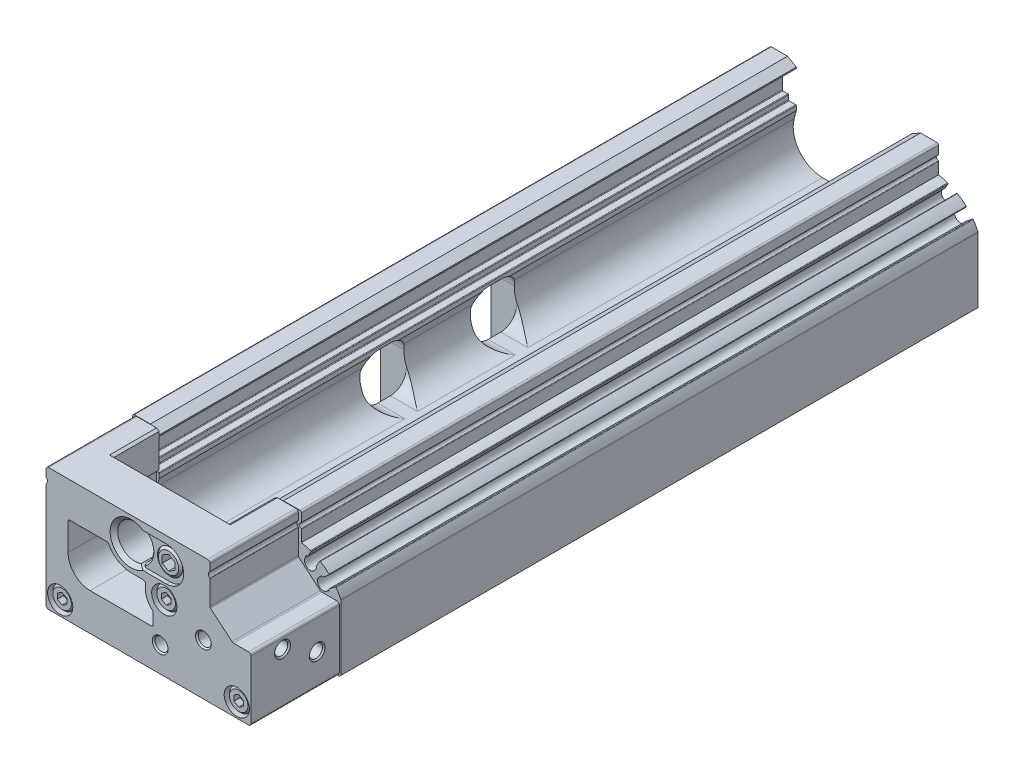
from build123d import *

# Parameters (mm, degrees)
BOSS_EXTRUDE1_DEPTH      = 28
BOSS_EXTRUDE2_DEPTH      = 202
CUT_EXTRUDE1_DEPTH       = 14.9
CUT_EXTRUDE2_DEPTH       = 8.7
BOSS_EXTRUDE3_START      = 7.5
BOSS_EXTRUDE3_DEPTH      = 7.5
BOSS_EXTRUDE4_DEPTH      = 8.7
CUT_EXTRUDE3_DEPTH       = 7.6
CUT_EXTRUDE3_DEPTH_BACK  = 7.6
CUT_EXTRUDE4_DEPTH       = 17
CUT_EXTRUDE5_DEPTH       = 7.6
CUT_EXTRUDE5_DEPTH_BACK  = 7.6
CUT_EXTRUDE6_DEPTH       = 17
CUT_EXTRUDE7_DEPTH       = 4.6
CUT_EXTRUDE7_DEPTH_BACK  = 4.6
SKETCH28_R               = 4
CUT_EXTRUDE8_DEPTH       = 4.6
CUT_EXTRUDE8_DEPTH_BACK  = 4.6
SKETCH29_R               = 4
CUT_EXTRUDE9_DEPTH       = 4.6
CUT_EXTRUDE9_DEPTH_BACK  = 4.6
SKETCH30_R               = 4
SKETCH33_W               = 8
SKETCH33_H               = 4
CUT_EXTRUDE10_DEPTH      = 5
CUT_EXTRUDE11_DEPTH      = 2
CUT_EXTRUDE11_DEPTH_BACK = 2
CUT_EXTRUDE12_DEPTH      = 2
CUT_EXTRUDE12_DEPTH_BACK = 2
CUT_EXTRUDE13_DEPTH      = 2
CUT_EXTRUDE13_DEPTH_BACK = 2


with BuildPart() as part:
    # Sketch1 → Boss-Extrude1 (new body)
    with BuildSketch(Plane.XY):
        with BuildLine():
            Line((0.8, 0), (64.2, 0))
            ThreePointArc((64.2, 0), (64.765685425, 0.234314575), (65, 0.8))
            Line((65, 0.8), (65, 19.3))
            ThreePointArc((65, 19.3), (64.765685425, 19.865685425), (64.2, 20.1))
            Line((64.2, 20.1), (59.464779164, 20.1))
            ThreePointArc((59.464779164, 20.1), (59.225365064, 20.142215165), (59.014827837, 20.26376889))
            Line((59.014827837, 20.26376889), (52.178606195, 26.000039948))
            ThreePointArc((52.178606195, 26.000039948), (52.046846106, 26.171753039), (52, 26.38306217))
            Line((52, 26.38306217), (52, 34.125320566))
            ThreePointArc((52, 34.125320566), (51.977951304, 34.216607658), (51.916666667, 34.287767138))
            ThreePointArc((51.916666667, 34.287767138), (51.5, 35.1), (51.916666667, 35.912232862))
            ThreePointArc((51.916666667, 35.912232862), (51.977951304, 35.983392342), (52, 36.074679434))
            Line((52, 36.074679434), (52, 38.2))
            ThreePointArc((52, 38.2), (51.765685425, 38.765685425), (51.2, 39))
            Line((51.2, 39), (0.8, 39))
            ThreePointArc((0.8, 39), (0.234314575, 38.765685425), (0, 38.2))
            Line((0, 38.2), (0, 36.074679434))
            ThreePointArc((0, 36.074679434), (0.022048696, 35.983392342), (0.083333333, 35.912232862))
            ThreePointArc((0.083333333, 35.912232862), (0.5, 35.1), (0.083333333, 34.287767138))
            ThreePointArc((0.083333333, 34.287767138), (0.022048696, 34.216607658), (0, 34.125320566))
            Line((0, 34.125320566), (0, 0.8))
            ThreePointArc((0, 0.8), (0.234314575, 0.234314575), (0.8, 0))
        make_face()
        with BuildLine():
            Line((7, 27.3), (7, 18.8))
            ThreePointArc((7, 18.8), (9.050252532, 13.850252532), (14, 11.8))
            Line((14, 11.8), (33.4, 11.8))
            ThreePointArc((33.4, 11.8), (33.824264069, 11.975735931), (34, 12.4))
            Line((34, 12.4), (34, 15.827959784))
            ThreePointArc((34, 15.827959784), (33.940201982, 16.089076268), (33.772727273, 16.298145258))
            ThreePointArc((33.772727273, 16.298145258), (31.893362377, 18.863270124), (31.588820692, 22.028571429))
            ThreePointArc((31.588820692, 22.028571429), (31.368943868, 22.843650304), (30.60362414, 23.2))
            Line((30.60362414, 23.2), (27, 23.2))
            ThreePointArc((27, 23.2), (22.818089899, 24.380056605), (19.869902457, 27.572093023))
            ThreePointArc((19.869902457, 27.572093023), (19.648788399, 27.811495755), (19.335145142, 27.9))
            Line((19.335145142, 27.9), (7.6, 27.9))
            ThreePointArc((7.6, 27.9), (7.175735931, 27.724264069), (7, 27.3))
        make_face(mode=Mode.SUBTRACT)
    extrude(amount=BOSS_EXTRUDE1_DEPTH)

    # Sketch2 → Boss-Extrude2 (add)
    with BuildSketch(Plane.XY):
        with BuildLine():
            Line((-0.5, 34.171291219), (-0.5, 0.25))
            Line((-0.5, 0.25), (0, -0.25))
            Line((0, -0.25), (7, -0.25))
            Line((7, -0.25), (7.25, -0.5))
            Line((7.25, -0.5), (45.15, -0.5))
            Line((45.15, -0.5), (45.4, -0.25))
            Line((45.4, -0.25), (65, -0.25))
            Line((65, -0.25), (65.5, 0.25))
            Line((65.5, 0.25), (65.5, 20.913874629))
            ThreePointArc((65.5, 20.913874629), (65.488140605, 21.022127805), (65.453125, 21.125245711))
            ThreePointArc((65.453125, 21.125245711), (64.780880489, 22.414771774), (63.997704608, 23.640098541))
            ThreePointArc((63.997704608, 23.640098541), (63.862603435, 23.723024943), (63.70959314, 23.681588675))
            Line((63.70959314, 23.681588675), (61.720720018, 22.09956756))
            ThreePointArc((61.720720018, 22.09956756), (61.646508574, 21.965686571), (61.688701313, 21.818543001))
            ThreePointArc((61.688701313, 21.818543001), (61.729316434, 21.660319143), (61.638419767, 21.524590836))
            Line((61.638419767, 21.524590836), (60.803979043, 21.001419089))
            ThreePointArc((60.803979043, 21.001419089), (58.439123592, 21.405935885), (58.576951262, 23.801176724))
            Line((58.576951262, 23.801176724), (59.274422472, 24.496542751))
            ThreePointArc((59.274422472, 24.496542751), (59.427119372, 24.554577516), (59.572151549, 24.479410735))
            ThreePointArc((59.572151549, 24.479410735), (59.706032538, 24.405199291), (59.853176108, 24.44739203))
            Line((59.853176108, 24.44739203), (61.721062189, 25.933175708))
            ThreePointArc((61.721062189, 25.933175708), (61.796411585, 26.082013006), (61.732713363, 26.236196693))
            ThreePointArc((61.732713363, 26.236196693), (60.422319434, 27.333230903), (59.00548184, 28.288839368))
            ThreePointArc((59.00548184, 28.288839368), (58.852359437, 28.311102038), (58.72918001, 28.217459497))
            Line((58.72918001, 28.217459497), (57.649038106, 26.346598839))
            ThreePointArc((57.649038106, 26.346598839), (57.629058021, 26.19483503), (57.722243186, 26.073393759))
            ThreePointArc((57.722243186, 26.073393759), (57.818021446, 25.941064993), (57.783194182, 25.781467252))
            Line((57.783194182, 25.781467252), (57.198558959, 24.988875518))
            ThreePointArc((57.198558959, 24.988875518), (54.85, 24.498522628), (54.10037858, 26.777610794))
            Line((54.10037858, 26.777610794), (54.494465545, 27.680215616))
            ThreePointArc((54.494465545, 27.680215616), (54.615267611, 27.790175782), (54.777756814, 27.773393759))
            ThreePointArc((54.777756814, 27.773393759), (54.929520623, 27.753413674), (55.050961894, 27.846598839))
            Line((55.050961894, 27.846598839), (55.982986307, 29.460912476))
            ThreePointArc((55.982986307, 29.460912476), (55.997122526, 29.630935595), (55.874931916, 29.750003426))
            ThreePointArc((55.874931916, 29.750003426), (54.453414575, 30.169379301), (53, 30.45950643))
            Line((53, 30.45950643), (53, 34.171291219))
            ThreePointArc((53, 34.171291219), (52.955597321, 34.296947391), (52.842105263, 34.366808857))
            ThreePointArc((52.842105263, 34.366808857), (52.25, 35.1), (52.842105263, 35.833191143))
            ThreePointArc((52.842105263, 35.833191143), (52.955597321, 35.903052609), (53, 36.028708781))
            Line((53, 36.028708781), (53, 38.6))
            ThreePointArc((53, 38.6), (52.853553391, 38.953553391), (52.5, 39.1))
            Line((52.5, 39.1), (47.271281292, 39.1))
            Line((47.271281292, 39.1), (44.5, 37.5))
            Line((44.5, 37.5), (44.5, 37.1))
            Line((44.5, 37.1), (48.95, 37.1))
            Line((48.95, 37.1), (48.95, 29.3))
            ThreePointArc((48.95, 29.3), (48.891421356, 29.158578644), (48.75, 29.1))
            Line((48.75, 29.1), (47.15, 29.1))
            ThreePointArc((47.15, 29.1), (47.008578644, 29.041421356), (46.95, 28.9))
            Line((46.95, 28.9), (46.95, 27.3))
            ThreePointArc((46.95, 27.3), (46.891421356, 27.158578644), (46.75, 27.1))
            Line((46.75, 27.1), (44.7, 27.1))
            ThreePointArc((44.7, 27.1), (44.558578644, 27.041421356), (44.5, 26.9))
            Line((44.5, 26.9), (44.5, 26.7))
            ThreePointArc((44.5, 26.7), (44.294974747, 26.205025253), (43.8, 26))
            Line((43.8, 26), (37.5, 26))
            ThreePointArc((37.5, 26), (35.025126266, 24.974873734), (34, 22.5))
            Line((34, 22.5), (34, 12.8))
            ThreePointArc((34, 12.8), (33.560660172, 11.739339828), (32.5, 11.3))
            Line((32.5, 11.3), (16.2, 11.3))
            ThreePointArc((16.2, 11.3), (8.821813935, 14.93851871), (7.216889816, 23.007017119))
            Line((7.216889816, 23.007017119), (7.9, 25.556419035))
            Line((7.9, 25.556419035), (7.9, 26.9))
            ThreePointArc((7.9, 26.9), (7.841421356, 27.041421356), (7.7, 27.1))
            Line((7.7, 27.1), (5.65, 27.1))
            ThreePointArc((5.65, 27.1), (5.508578644, 27.158578644), (5.45, 27.3))
            Line((5.45, 27.3), (5.45, 28.65))
            ThreePointArc((5.45, 28.65), (5.391421356, 28.791421356), (5.25, 28.85))
            Line((5.25, 28.85), (3.65, 28.85))
            ThreePointArc((3.65, 28.85), (3.508578644, 28.908578644), (3.45, 29.05))
            Line((3.45, 29.05), (3.45, 37.1))
            Line((3.45, 37.1), (7.9, 37.1))
            Line((7.9, 37.1), (7.9, 37.5))
            Line((7.9, 37.5), (5.128718708, 39.1))
            Line((5.128718708, 39.1), (0, 39.1))
            ThreePointArc((0, 39.1), (-0.353553391, 38.953553391), (-0.5, 38.6))
            Line((-0.5, 38.6), (-0.5, 36.028708781))
            ThreePointArc((-0.5, 36.028708781), (-0.455597321, 35.903052609), (-0.342105263, 35.833191143))
            ThreePointArc((-0.342105263, 35.833191143), (0.25, 35.1), (-0.342105263, 34.366808857))
            ThreePointArc((-0.342105263, 34.366808857), (-0.455597321, 34.296947391), (-0.5, 34.171291219))
        make_face()
    extrude(amount=-BOSS_EXTRUDE2_DEPTH)

    # Sketch3 → Cut-Extrude1 (cut)
    with BuildSketch(Plane.XY):
        with BuildLine():
            Line((7.033974596, 39), (7.9, 38.5))
            Line((7.9, 38.5), (7.9, 18.8))
            ThreePointArc((7.9, 18.8), (9.950252532, 13.850252532), (14.9, 11.8))
            Line((14.9, 11.8), (33, 11.8))
            ThreePointArc((33, 11.8), (33.707106781, 12.092893219), (34, 12.8))
            Line((34, 12.8), (34, 23))
            ThreePointArc((34, 23), (34.878679656, 25.121320344), (37, 26))
            Line((37, 26), (41.5, 26))
            ThreePointArc((41.5, 26), (46.24341649, 29.41886117), (44.5, 35))
            Line((44.5, 35), (44.5, 38.5))
            Line((44.5, 38.5), (45.366025404, 39))
            Line((45.366025404, 39), (7.033974596, 39))
        make_face()
    extrude(amount=CUT_EXTRUDE1_DEPTH, mode=Mode.SUBTRACT)

    # Sketch4 → Cut-Extrude2 (cut)
    with BuildSketch(Plane.XY.offset(28)):
        with BuildLine():
            Line((31.15, 25.7), (38.15, 25.7))
            ThreePointArc((38.15, 25.7), (43.65, 31.2), (38.15, 36.7))
            Line((38.15, 36.7), (31.15, 36.7))
            ThreePointArc((31.15, 36.7), (25.65, 31.2), (31.15, 25.7))
        make_face()
    extrude(amount=-CUT_EXTRUDE2_DEPTH, mode=Mode.SUBTRACT)

    # Sketch5 → Boss-Extrude3 (add)
    with BuildSketch(Plane.XY.offset(19.3).offset(BOSS_EXTRUDE3_START)):
        with BuildLine():
            Line((30.15, 25.7), (38.15, 25.7))
            ThreePointArc((38.15, 25.7), (43.65, 31.2), (38.15, 36.7))
            Line((38.15, 36.7), (30.15, 36.7))
            Line((30.15, 36.7), (30.15, 25.7))
        make_face()
    extrude(amount=-BOSS_EXTRUDE3_DEPTH)

    # Sketch6 → Cut-Revolve1 (revolve, cut)
    with BuildSketch(Plane(origin=(0, 31.2, 0), x_dir=(1, 0, 0), z_dir=(0, 1, 0))):
        Polygon((27, -19.3), (31.8, -19.3), (31.8, -25.6), (33, -26.8), (27, -26.8), align=None)
    revolve(axis=Axis((27, 31.2, 26.8), (0, 0, -1)), mode=Mode.SUBTRACT)

    # Sketch7 → Boss-Extrude4 (add)
    with BuildSketch(Plane.XY.offset(28)):
        with BuildLine():
            Line((27, 25.2), (31.15, 25.2))
            Line((31.15, 25.2), (31.15, 25.7))
            ThreePointArc((31.15, 25.7), (25.65, 31.2), (31.15, 36.7))
            Line((31.15, 36.7), (31.15, 37.2))
            Line((31.15, 37.2), (27, 37.2))
            ThreePointArc((27, 37.2), (21, 31.2), (27, 25.2))
        make_face()
    extrude(amount=-BOSS_EXTRUDE4_DEPTH)

    # Sketch8 → Cut-Revolve2 (revolve, cut)
    with BuildSketch(Plane(origin=(27, 0, 0), x_dir=(0, 0, -1), z_dir=(1, 0, 0)), mode=Mode.PRIVATE) as cut_revolve2_sk:
        Polygon((-14.9, 31.2), (-14.9, 25.7415), (-26.8, 25.7415), (-28, 24.5415), (-28, 31.2), align=None)
    revolve(cut_revolve2_sk.sketch.rotate(Axis((27, 31.2, 28), (0, 0, -1)), 90), axis=Axis((27, 31.2, 28), (0, 0, -1)), mode=Mode.SUBTRACT)

    # Sketch9 → Cut-Revolve3 (revolve, cut)
    with BuildSketch(Plane(origin=(36.2, 0, 0), x_dir=(0, 0, -1), z_dir=(1, 0, 0)), mode=Mode.PRIVATE) as cut_revolve3_sk:
        Polygon((-28, 8), (-28, 10.5), (-27.567, 10.067), (-5.1, 10.067), (-3.906616994, 8), align=None)
    revolve(cut_revolve3_sk.sketch.rotate(Axis((36.2, 8, 3.906616994), (0, 0, 1)), 270), axis=Axis((36.2, 8, 3.906616994), (0, 0, 1)), mode=Mode.SUBTRACT)

    # Sketch10 → Cut-Revolve4 (revolve, cut)
    with BuildSketch(Plane(origin=(49.9, 0, 0), x_dir=(0, 0, -1), z_dir=(1, 0, 0)), mode=Mode.PRIVATE) as cut_revolve4_sk:
        Polygon((-28, 16.2), (-28, 18.7), (-27.567, 18.267), (-7, 18.267), (-5.806616994, 16.2), align=None)
    revolve(cut_revolve4_sk.sketch.rotate(Axis((49.9, 16.2, 5.806616994), (0, 0, 1)), 270), axis=Axis((49.9, 16.2, 5.806616994), (0, 0, 1)), mode=Mode.SUBTRACT)

    # Sketch11 → Cut-Extrude3 (cut, two sides: drawn at the far end of the back side and taken through both)
    with BuildSketch(Plane(origin=(0, 0, 0), x_dir=(0, 0, -1), z_dir=(1, 0, 0)).offset(-CUT_EXTRUDE3_DEPTH_BACK)):
        with BuildLine():
            Line((99.6, 21.1), (99.6, -0.5))
            Line((99.6, -0.5), (113.6, -0.5))
            Line((113.6, -0.5), (113.6, 21.1))
            ThreePointArc((113.6, 21.1), (112.135533906, 24.635533906), (108.6, 26.1))
            Line((108.6, 26.1), (104.6, 26.1))
            ThreePointArc((104.6, 26.1), (101.064466094, 24.635533906), (99.6, 21.1))
        make_face()
    extrude(amount=CUT_EXTRUDE3_DEPTH + CUT_EXTRUDE3_DEPTH_BACK, mode=Mode.SUBTRACT)

    # Sketch12 → Cut-Extrude4 (cut)
    with BuildSketch(Plane(origin=(0, 0, 0), x_dir=(0, 0, -1), z_dir=(1, 0, 0))):
        with BuildLine():
            Line((104.6, 11.3), (108.6, 11.3))
            ThreePointArc((108.6, 11.3), (112.135533906, 12.764466094), (113.6, 16.3))
            Line((113.6, 16.3), (113.6, 21.1))
            ThreePointArc((113.6, 21.1), (112.135533906, 24.635533906), (108.6, 26.1))
            Line((108.6, 26.1), (104.6, 26.1))
            ThreePointArc((104.6, 26.1), (101.064466094, 24.635533906), (99.6, 21.1))
            Line((99.6, 21.1), (99.6, 16.3))
            ThreePointArc((99.6, 16.3), (101.064466094, 12.764466094), (104.6, 11.3))
        make_face()
    extrude(amount=CUT_EXTRUDE4_DEPTH, mode=Mode.SUBTRACT)

    # Sketch13 → Cut-Extrude5 (cut, two sides: drawn at the far end of the back side and taken through both)
    with BuildSketch(Plane(origin=(0, 0, 0), x_dir=(0, 0, -1), z_dir=(1, 0, 0)).offset(-CUT_EXTRUDE5_DEPTH_BACK)):
        with BuildLine():
            Line((64.6, 21.1), (64.6, -0.5))
            Line((64.6, -0.5), (78.6, -0.5))
            Line((78.6, -0.5), (78.6, 21.1))
            ThreePointArc((78.6, 21.1), (77.135533906, 24.635533906), (73.6, 26.1))
            Line((73.6, 26.1), (69.6, 26.1))
            ThreePointArc((69.6, 26.1), (66.064466094, 24.635533906), (64.6, 21.1))
        make_face()
    extrude(amount=CUT_EXTRUDE5_DEPTH + CUT_EXTRUDE5_DEPTH_BACK, mode=Mode.SUBTRACT)

    # Sketch14 → Cut-Extrude6 (cut)
    with BuildSketch(Plane(origin=(0, 0, 0), x_dir=(0, 0, -1), z_dir=(1, 0, 0))):
        with BuildLine():
            Line((69.6, 11.3), (73.6, 11.3))
            ThreePointArc((73.6, 11.3), (77.135533906, 12.764466094), (78.6, 16.3))
            Line((78.6, 16.3), (78.6, 21.1))
            ThreePointArc((78.6, 21.1), (77.135533906, 24.635533906), (73.6, 26.1))
            Line((73.6, 26.1), (69.6, 26.1))
            ThreePointArc((69.6, 26.1), (66.064466094, 24.635533906), (64.6, 21.1))
            Line((64.6, 21.1), (64.6, 16.3))
            ThreePointArc((64.6, 16.3), (66.064466094, 12.764466094), (69.6, 11.3))
        make_face()
    extrude(amount=CUT_EXTRUDE6_DEPTH, mode=Mode.SUBTRACT)

    # Sketch15 → Cut-Revolve5 (revolve, cut)
    with BuildSketch(Plane(origin=(0, 10, 0), x_dir=(1, 0, 0), z_dir=(0, 1, 0))):
        Polygon((34.806616994, -7), (36, -4.933), (64.567, -4.933), (65, -4.5), (65, -7), align=None)
    revolve(axis=Axis((65, 10, 7), (-1, 0, 0)), mode=Mode.SUBTRACT)

    # Sketch16 → Cut-Revolve6 (revolve, cut)
    with BuildSketch(Plane(origin=(0, 16.2, 0), x_dir=(1, 0, 0), z_dir=(0, 1, 0)), mode=Mode.PRIVATE) as cut_revolve6_sk:
        Polygon((49.606616994, -18), (50.8, -15.933), (64.567, -15.933), (65, -15.5), (65, -18), align=None)
    revolve(cut_revolve6_sk.sketch.rotate(Axis((65, 16.2, 18), (-1, 0, 0)), 180), axis=Axis((65, 16.2, 18), (-1, 0, 0)), mode=Mode.SUBTRACT)

    # Sketch17 → Cut-Revolve7 (revolve, cut)
    with BuildSketch(Plane(origin=(48.5, 0, 0), x_dir=(0, 0, -1), z_dir=(1, 0, 0)), mode=Mode.PRIVATE) as cut_revolve7_sk:
        Polygon((83.6, 13.5), (83.6, 23.5), (193.6, 23.5), (193.6, 17.5), (194.1, 17.5), (194.1, 19.5), (202, 19.5), (202, 13.5), align=None)
    revolve(cut_revolve7_sk.sketch.rotate(Axis((48.5, 13.5, -202), (0, 0, 1)), 270), axis=Axis((48.5, 13.5, -202), (0, 0, 1)), mode=Mode.SUBTRACT)

    # Sketch18 → Cut-Revolve8 (revolve, cut)
    with BuildSketch(Plane(origin=(26.2, 0, 0), x_dir=(0, 0, -1), z_dir=(1, 0, 0)), mode=Mode.PRIVATE) as cut_revolve8_sk:
        Polygon((196.5, 11.3), (199, 11.3), (198.567, 10.867), (198.567, 1.533), (199, 1.1), (200, 1.1), (200, -0.5), (196.5, -0.5), align=None)
    revolve(cut_revolve8_sk.sketch.rotate(Axis((26.2, -0.5, -196.5), (0, 1, 0)), 180), axis=Axis((26.2, -0.5, -196.5), (0, 1, 0)), mode=Mode.SUBTRACT)

    # Sketch19 → Cut-Revolve9 (revolve, cut)
    with BuildSketch(Plane(origin=(26.2, 0, 0), x_dir=(0, 0, -1), z_dir=(1, 0, 0)), mode=Mode.PRIVATE) as cut_revolve9_sk:
        Polygon((186.5, 11.3), (189, 11.3), (188.567, 10.867), (188.567, 1.533), (189, 1.1), (190, 1.1), (190, -0.5), (186.5, -0.5), align=None)
    revolve(cut_revolve9_sk.sketch.rotate(Axis((26.2, -0.5, -186.5), (0, 1, 0)), 180), axis=Axis((26.2, -0.5, -186.5), (0, 1, 0)), mode=Mode.SUBTRACT)

    # Sketch20 → Cut-Revolve10 (revolve, cut)
    with BuildSketch(Plane(origin=(26.2, 0, 0), x_dir=(0, 0, -1), z_dir=(1, 0, 0)), mode=Mode.PRIVATE) as cut_revolve10_sk:
        Polygon((176.5, 16.3), (181, 16.3), (181, 5.6), (179.25, 5.6), (179.25, 1.1), (180, 1.1), (180, -0.5), (176.5, -0.5), align=None)
    revolve(cut_revolve10_sk.sketch.rotate(Axis((26.2, -0.5, -176.5), (0, 1, 0)), 180), axis=Axis((26.2, -0.5, -176.5), (0, 1, 0)), mode=Mode.SUBTRACT)

    # Sketch21 → Cut-Revolve11 (revolve, cut)
    with BuildSketch(Plane(origin=(26.2, 0, 0), x_dir=(0, 0, -1), z_dir=(1, 0, 0)), mode=Mode.PRIVATE) as cut_revolve11_sk:
        Polygon((166.5, 16.3), (171, 16.3), (171, 5.6), (169.25, 5.6), (169.25, 1.1), (170, 1.1), (170, -0.5), (166.5, -0.5), align=None)
    revolve(cut_revolve11_sk.sketch.rotate(Axis((26.2, -0.5, -166.5), (0, 1, 0)), 180), axis=Axis((26.2, -0.5, -166.5), (0, 1, 0)), mode=Mode.SUBTRACT)

    # Sketch22 → Cut-Revolve12 (revolve, cut)
    with BuildSketch(Plane(origin=(26.2, 0, 0), x_dir=(0, 0, -1), z_dir=(1, 0, 0)), mode=Mode.PRIVATE) as cut_revolve12_sk:
        Polygon((156.5, 16.3), (161, 16.3), (161, 5.6), (159.25, 5.6), (159.25, 1.1), (160, 1.1), (160, -0.5), (156.5, -0.5), align=None)
    revolve(cut_revolve12_sk.sketch.rotate(Axis((26.2, -0.5, -156.5), (0, 1, 0)), 180), axis=Axis((26.2, -0.5, -156.5), (0, 1, 0)), mode=Mode.SUBTRACT)

    # Sketch23 → Cut-Revolve13 (revolve, cut)
    with BuildSketch(Plane(origin=(26.2, 0, 0), x_dir=(0, 0, -1), z_dir=(1, 0, 0)), mode=Mode.PRIVATE) as cut_revolve13_sk:
        Polygon((146.5, 11.3), (149, 11.3), (148.567, 10.867), (148.567, 1.533), (149, 1.1), (150, 1.1), (150, -0.5), (146.5, -0.5), align=None)
    revolve(cut_revolve13_sk.sketch.rotate(Axis((26.2, -0.5, -146.5), (0, 1, 0)), 180), axis=Axis((26.2, -0.5, -146.5), (0, 1, 0)), mode=Mode.SUBTRACT)

    # Sketch24 → Cut-Revolve14 (revolve, cut)
    with BuildSketch(Plane(origin=(26.2, 0, 0), x_dir=(0, 0, -1), z_dir=(1, 0, 0)), mode=Mode.PRIVATE) as cut_revolve14_sk:
        Polygon((136.5, 11.3), (139, 11.3), (138.567, 10.867), (138.567, 1.533), (139, 1.1), (140, 1.1), (140, -0.5), (136.5, -0.5), align=None)
    revolve(cut_revolve14_sk.sketch.rotate(Axis((26.2, -0.5, -136.5), (0, 1, 0)), 180), axis=Axis((26.2, -0.5, -136.5), (0, 1, 0)), mode=Mode.SUBTRACT)

    # Sketch25 → Cut-Revolve15 (revolve, cut)
    with BuildSketch(Plane(origin=(26.2, 0, 0), x_dir=(0, 0, -1), z_dir=(1, 0, 0)), mode=Mode.PRIVATE) as cut_revolve15_sk:
        Polygon((126.5, 16.3), (131, 16.3), (131, 5.6), (129.25, 5.6), (129.25, 1.1), (130, 1.1), (130, -0.5), (126.5, -0.5), align=None)
    revolve(cut_revolve15_sk.sketch.rotate(Axis((26.2, -0.5, -126.5), (0, 1, 0)), 180), axis=Axis((26.2, -0.5, -126.5), (0, 1, 0)), mode=Mode.SUBTRACT)

    # Sketch26 → Cut-Revolve16 (revolve, cut)
    with BuildSketch(Plane(origin=(26.2, 0, 0), x_dir=(0, 0, -1), z_dir=(1, 0, 0)), mode=Mode.PRIVATE) as cut_revolve16_sk:
        Polygon((116.5, 16.3), (121, 16.3), (121, 5.6), (119.25, 5.6), (119.25, 1.1), (120, 1.1), (120, -0.5), (116.5, -0.5), align=None)
    revolve(cut_revolve16_sk.sketch.rotate(Axis((26.2, -0.5, -116.5), (0, 1, 0)), 180), axis=Axis((26.2, -0.5, -116.5), (0, 1, 0)), mode=Mode.SUBTRACT)

    # Sketch27 → Cut-Revolve17 (revolve, cut)
    with BuildSketch(Plane(origin=(26.2, 0, 0), x_dir=(0, 0, -1), z_dir=(1, 0, 0)), mode=Mode.PRIVATE) as cut_revolve17_sk:
        Polygon((106.5, 16.3), (111, 16.3), (111, 5.6), (109.25, 5.6), (109.25, 1.1), (110, 1.1), (110, -0.5), (106.5, -0.5), align=None)
    revolve(cut_revolve17_sk.sketch.rotate(Axis((26.2, -0.5, -106.5), (0, 1, 0)), 180), axis=Axis((26.2, -0.5, -106.5), (0, 1, 0)), mode=Mode.SUBTRACT)

    # Sketch28 → Cut-Extrude7 (cut, two sides: drawn at the far end of the back side and taken through both)
    with BuildSketch(Plane.XY.offset(28).offset(-CUT_EXTRUDE7_DEPTH_BACK)):
        with Locations((60.5, 4.5)):
            Circle(SKETCH28_R)
    extrude(amount=CUT_EXTRUDE7_DEPTH + CUT_EXTRUDE7_DEPTH_BACK, mode=Mode.SUBTRACT)

    # Sketch29 → Cut-Extrude8 (cut, two sides: drawn at the far end of the back side and taken through both)
    with BuildSketch(Plane.XY.offset(28).offset(-CUT_EXTRUDE8_DEPTH_BACK)):
        with Locations((4.5, 4.5)):
            Circle(SKETCH29_R)
    extrude(amount=CUT_EXTRUDE8_DEPTH + CUT_EXTRUDE8_DEPTH_BACK, mode=Mode.SUBTRACT)

    # Sketch30 → Cut-Extrude9 (cut, two sides: drawn at the far end of the back side and taken through both)
    with BuildSketch(Plane.XY.offset(28).offset(-CUT_EXTRUDE9_DEPTH_BACK)):
        with Locations((37.5, 21)):
            Circle(SKETCH30_R)
    extrude(amount=CUT_EXTRUDE9_DEPTH + CUT_EXTRUDE9_DEPTH_BACK, mode=Mode.SUBTRACT)

    # Sketch31 → Revolve1 (revolve)
    with BuildSketch(Plane(origin=(4.5, 0, 0), x_dir=(0, 0, -1), z_dir=(1, 0, 0)), mode=Mode.PRIVATE) as revolve1_sk:
        Polygon((-27.4, 4.5), (-27.4, 7.428571429), (-26.828571429, 8), (-23.4, 8), (-23.4, 4.5), align=None)
    revolve(revolve1_sk.sketch.rotate(Axis((4.5, 4.5, 23.4), (0, 0, 1)), 270), axis=Axis((4.5, 4.5, 23.4), (0, 0, 1)))

    # Sketch33 → Cut-Revolve18 (revolve, cut)
    with BuildSketch(Plane(origin=(38.15, 0, 0), x_dir=(0, 0, -1), z_dir=(1, 0, 0)), mode=Mode.PRIVATE) as cut_revolve18_sk:
        with Locations((-24.3, 29.2)):
            Rectangle(SKETCH33_W, SKETCH33_H)
    revolve(cut_revolve18_sk.sketch.rotate(Axis((38.15, 31.2, 28.3), (0, 0, -1)), 90), axis=Axis((38.15, 31.2, 28.3), (0, 0, -1)), mode=Mode.SUBTRACT)

    # Sketch32 → Revolve2 (revolve)
    with BuildSketch(Plane(origin=(38.15, 0, 0), x_dir=(0, 0, -1), z_dir=(1, 0, 0)), mode=Mode.PRIVATE) as revolve2_sk:
        Polygon((-19.3, 31.2), (-19.3, 27.2), (-26.5, 27.2), (-27.3, 28), (-27.3, 31.2), align=None)
    revolve(revolve2_sk.sketch.rotate(Axis((38.15, 31.2, 27.3), (0, 0, -1)), 90), axis=Axis((38.15, 31.2, 27.3), (0, 0, -1)))

    # Sketch34 → Cut-Extrude10 (cut)
    with BuildSketch(Plane.XY.offset(27.3)):
        Polygon((36.15, 30.045299462), (38.15, 28.890598923), (40.15, 30.045299462), (40.15, 32.354700538), (38.15, 33.509401077), (36.15, 32.354700538), align=None)
    extrude(amount=-CUT_EXTRUDE10_DEPTH, mode=Mode.SUBTRACT)

    # Sketch35 → Cut-Revolve19 (revolve, cut)
    with BuildSketch(Plane.XY.offset(18), mode=Mode.PRIVATE) as cut_revolve19_sk:
        Polygon((0, 34), (0, 35.5), (0.2705, 35.2295), (8, 35.2295), (8.709852156, 34), align=None)
    revolve(cut_revolve19_sk.sketch.rotate(Axis((8.709852156, 34, 18), (-1, 0, 0)), 270), axis=Axis((8.709852156, 34, 18), (-1, 0, 0)), mode=Mode.SUBTRACT)

    # Sketch36 → Revolve3 (revolve)
    with BuildSketch(Plane(origin=(37.5, 0, 0), x_dir=(0, 0, -1), z_dir=(1, 0, 0)), mode=Mode.PRIVATE) as revolve3_sk:
        Polygon((-27.4, 21), (-27.4, 23.928571429), (-26.828571429, 24.5), (-23.4, 24.5), (-23.4, 21), align=None)
    revolve(revolve3_sk.sketch.rotate(Axis((37.5, 21, 23.4), (0, 0, 1)), 270), axis=Axis((37.5, 21, 23.4), (0, 0, 1)))

    # Sketch37 → Revolve4 (revolve)
    with BuildSketch(Plane(origin=(60.5, 0, 0), x_dir=(0, 0, -1), z_dir=(1, 0, 0)), mode=Mode.PRIVATE) as revolve4_sk:
        Polygon((-27.4, 4.5), (-27.4, 7.428571429), (-26.828571429, 8), (-23.4, 8), (-23.4, 4.5), align=None)
    revolve(revolve4_sk.sketch.rotate(Axis((60.5, 4.5, 23.4), (0, 0, 1)), 270), axis=Axis((60.5, 4.5, 23.4), (0, 0, 1)))

    # Sketch38 → Cut-Extrude11 (cut, two sides: drawn at the far end of the back side and taken through both)
    with BuildSketch(Plane.XY.offset(27.4).offset(-CUT_EXTRUDE11_DEPTH_BACK)):
        Polygon((59, 3.633974596), (60.5, 2.767949192), (62, 3.633974596), (62, 5.366025404), (60.5, 6.232050808), (59, 5.366025404), align=None)
    extrude(amount=CUT_EXTRUDE11_DEPTH + CUT_EXTRUDE11_DEPTH_BACK, mode=Mode.SUBTRACT)

    # Sketch39 → Cut-Extrude12 (cut, two sides: drawn at the far end of the back side and taken through both)
    with BuildSketch(Plane.XY.offset(27.4).offset(-CUT_EXTRUDE12_DEPTH_BACK)):
        Polygon((3, 3.633974596), (4.5, 2.767949192), (6, 3.633974596), (6, 5.366025404), (4.5, 6.232050808), (3, 5.366025404), align=None)
    extrude(amount=CUT_EXTRUDE12_DEPTH + CUT_EXTRUDE12_DEPTH_BACK, mode=Mode.SUBTRACT)

    # Sketch40 → Cut-Revolve20 (revolve, cut)
    with BuildSketch(Plane.XY.offset(-106.6), mode=Mode.PRIVATE) as cut_revolve20_sk:
        Polygon((7.6, 6.5), (7.6, 9), (8.033, 8.567), (20.3, 8.567), (21.493383006, 6.5), align=None)
    revolve(cut_revolve20_sk.sketch.rotate(Axis((21.493383006, 6.5, -106.6), (-1, 0, 0)), 270), axis=Axis((21.493383006, 6.5, -106.6), (-1, 0, 0)), mode=Mode.SUBTRACT)

    # Sketch41 → Cut-Revolve21 (revolve, cut)
    with BuildSketch(Plane.XY.offset(-71.6), mode=Mode.PRIVATE) as cut_revolve21_sk:
        Polygon((7.6, 6.5), (7.6, 9), (8.033, 8.567), (20.3, 8.567), (21.493383006, 6.5), align=None)
    revolve(cut_revolve21_sk.sketch.rotate(Axis((21.493383006, 6.5, -71.6), (-1, 0, 0)), 270), axis=Axis((21.493383006, 6.5, -71.6), (-1, 0, 0)), mode=Mode.SUBTRACT)

    # Sketch42 → Cut-Extrude13 (cut, two sides: drawn at the far end of the back side and taken through both)
    with BuildSketch(Plane.XY.offset(27.4).offset(-CUT_EXTRUDE13_DEPTH_BACK)):
        Polygon((36, 20.133974596), (37.5, 19.267949192), (39, 20.133974596), (39, 21.866025404), (37.5, 22.732050808), (36, 21.866025404), align=None)
    extrude(amount=CUT_EXTRUDE13_DEPTH + CUT_EXTRUDE13_DEPTH_BACK, mode=Mode.SUBTRACT)


solid = part.part
